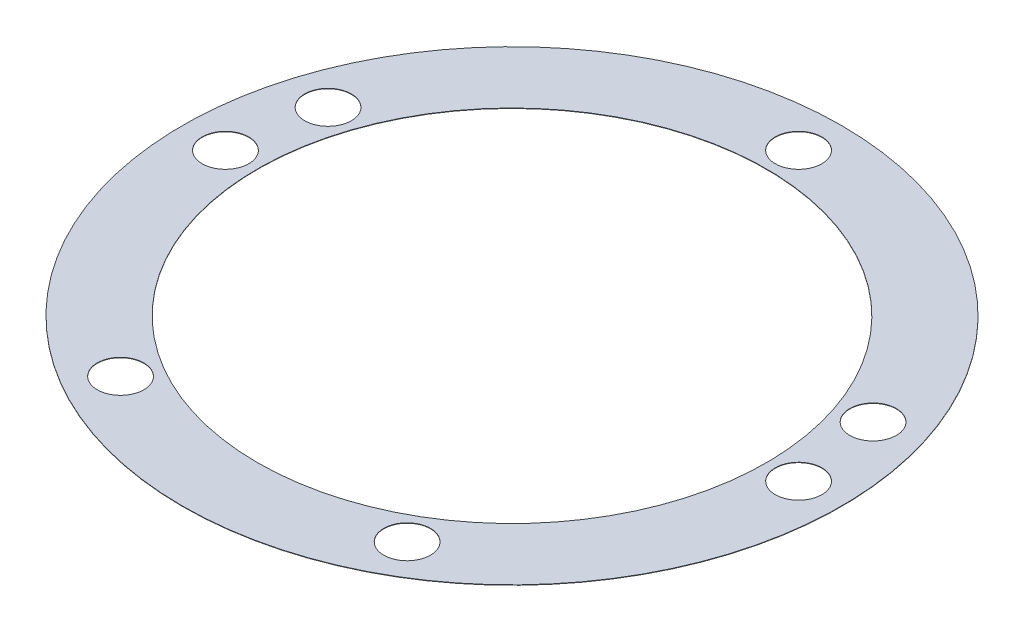
SolidWorks part; units mm, degrees
material "瓦楞纸"
ref_plane "Front Plane" through (0, 0, 0) normal (0, 0, 1) x (1, 0, 0)
ref_plane "Top Plane" through (0, 0, 0) normal (0, 1, 0) x (1, 0, 0)
ref_plane "Right Plane" through (0, 0, 0) normal (1, 0, 0) x (0, 0, -1)
sketch "Sketch1" plane through (0, 0, 0) normal (0, 1, 0) x (1, 0, 0)
  circle A0 centre (0, 0) radius 146.05
  circle A1 centre (0, 0) radius 112.776
  dimension "D1" = 292.1
  dimension "D2" = 225.552
extrude "Boss-Extrude1" add sketch "Sketch1" along normal blind 0.1778
hole_wizard "13/16 (0.8125) Diameter Hole1" positions "Sketch3" profile "Sketch2" hole size "13/16" standard "Ansi Inch" end condition through all
sketch "Sketch3" plane through (0, 0.1778, 0) normal (0, 1, 0) x (1, 0, 0)
  line L0 (0, -55) -> (0, 55) construction
  line L1 (-55, 0) -> (55, 0) construction
  point P0 (0, 127)
  dimension "D1" = 0
  dimension "D2" = 127
sketch "Sketch2" plane through (0, 0.1778, -127) normal (1, 0, 0) x (0, 0, 1)
  line L0 (0, 0) -> (0, 0.1778)
  line L1 (0, 0.1778) -> (10.3187, 0.1778)
  line L2 (10.3187, 0.1778) -> (10.3187, 0)
  line L5 (10.3187, 0) -> (0, 0)
  line L11 (0, -6.35) -> (0, 107.95) construction
  dimension "通孔孔直径" = 20.6375
  dimension "通孔孔深度" = 0.1778
hole_wizard "13/16 (0.8125) Diameter Hole2" positions "Sketch5" profile "Sketch4" hole size "13/16" standard "Ansi Inch" end condition through all
sketch "Sketch5" plane through (0, 0, 0) normal (0, -1, 0) x (-1, 0, 0)
  line L0 (-55, 0) -> (55, 0) construction
  line L1 (0, 55) -> (0, -55) construction
  point P0 (-63.5, -109.982)
  point P2 (-120.77, 39.243)
  point P9 (-127, 0)
  dimension "D1" = 109.982
  dimension "D2" = 63.5
  dimension "D3" = 39.243
  dimension "D4" = 120.77
  dimension "D5" = 0
  dimension "D6" = 127
sketch "Sketch4" plane through (63.5, 0, 109.982) normal (1, 0, 0) x (0, 0, -1)
  line L0 (0, 0) -> (0, 0.1778)
  line L1 (0, 0.1778) -> (10.3187, 0.1778)
  line L2 (10.3187, 0.1778) -> (10.3187, 0)
  line L5 (10.3187, 0) -> (0, 0)
  line L11 (0, -6.35) -> (0, 107.95) construction
  dimension "通孔孔直径" = 20.6375
  dimension "通孔孔深度" = 0.1778
mirror "Mirror1" about plane through (0, 0, 0) normal (1, 0, 0) of "13/16 (0.8125) Diameter Hole2"
